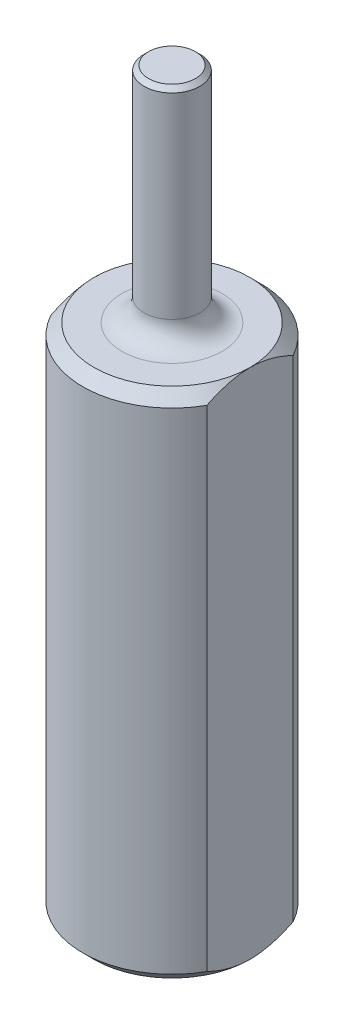
SolidWorks part; units mm, degrees
material "AL6061"
ref_plane "前视基准面" through (0, 0, 0) normal (0, 0, 1) x (1, 0, 0)
ref_plane "上视基准面" through (0, 0, 0) normal (0, 1, 0) x (1, 0, 0)
ref_plane "右视基准面" through (0, 0, 0) normal (1, 0, 0) x (0, 0, -1)
sketch "草图1" plane through (0, 0, 0) normal (0, 0, 1) x (1, 0, 0)
  line L0 (0, -0.5244) -> (0, 31.2009) construction
  line L1 (1.25, 33) -> (1.25, 23)
  line L2 (0, 0) -> (4, 0)
  line L3 (0, 0) -> (0, 33)
  line L4 (0, 33) -> (1.25, 33)
  line L5 (4, 0) -> (4, 23)
  line L6 (1.25, 23) -> (4, 23)
  dimension "D1" = 8
  dimension "D2" = 33
  dimension "D3" = 2.5
  dimension "D4" = 23
revolve "旋转1" add sketch "草图1" angle 360 about L0
hole_wizard "M3 螺纹孔1" positions "草图2" profile "草图3" tap size "M3" standard "GB"
sketch "草图2" plane through (0, 0, 0) normal (0, -1, 0) x (-1, 0, 0)
  point P0 (0, 0)
sketch "草图3" plane through (0, 0, 0) normal (1, 0, 0) x (0, 0, -1)
  line L0 (0, 0) -> (0, 12.2511)
  line L1 (0, 12.2511) -> (1.25, 11.5)
  line L2 (1.25, 11.5) -> (1.25, 0)
  line L5 (1.25, 0) -> (0, 0)
  line L10 (0, 12.2511) -> (-1.25, 11.5) construction
  line L11 (0, -6.35) -> (0, 107.95) construction
  dimension "螺纹孔钻头直径" = 2.5
  dimension "螺纹孔钻头深度" = 11.5
  dimension "导头角度" = 118
cosmetic thread "孔螺蚊线1" parameters "D1"=10, "D2"=3
chamfer "倒角1" distance 0.5 angle 45 2 edges at (0, 0, -4) (0, 23, -4)
fillet "圆角1" radius 1 1 edges at (0, 23, -1.25)
sketch "草图4" plane through (0, 0, 0) normal (0, 0, 1) x (1, 0, 0)
  line L0 (0, 31.0004) -> (0, -0.4978) construction
  line L1 (3.5, 23) -> (-3.5, 23) construction
  line L2 (3.5, 23) -> (4, 23)
  line L3 (3.5, 23) -> (3.5, 0)
  line L4 (3.5, 0) -> (4, 0)
  line L5 (4, 23) -> (4, 0)
  line L6 (4, 0.5) -> (4, 22.5) construction
  line L7 (-3.5, 0) -> (3.5, 0) construction
  line L8 (-4, 23) -> (-4, 0)
  line L9 (-3.5, 0) -> (-4, 0)
  line L10 (-3.5, 23) -> (-3.5, 0)
  line L11 (-3.5, 23) -> (-4, 23)
  dimension "D1" = 0.5
extrude "切除-拉伸1" cut sketch "草图4" against normal mid plane 10
chamfer "倒角2" distance 0.2 angle 45 1 edges at (0, 33, -1.25)
